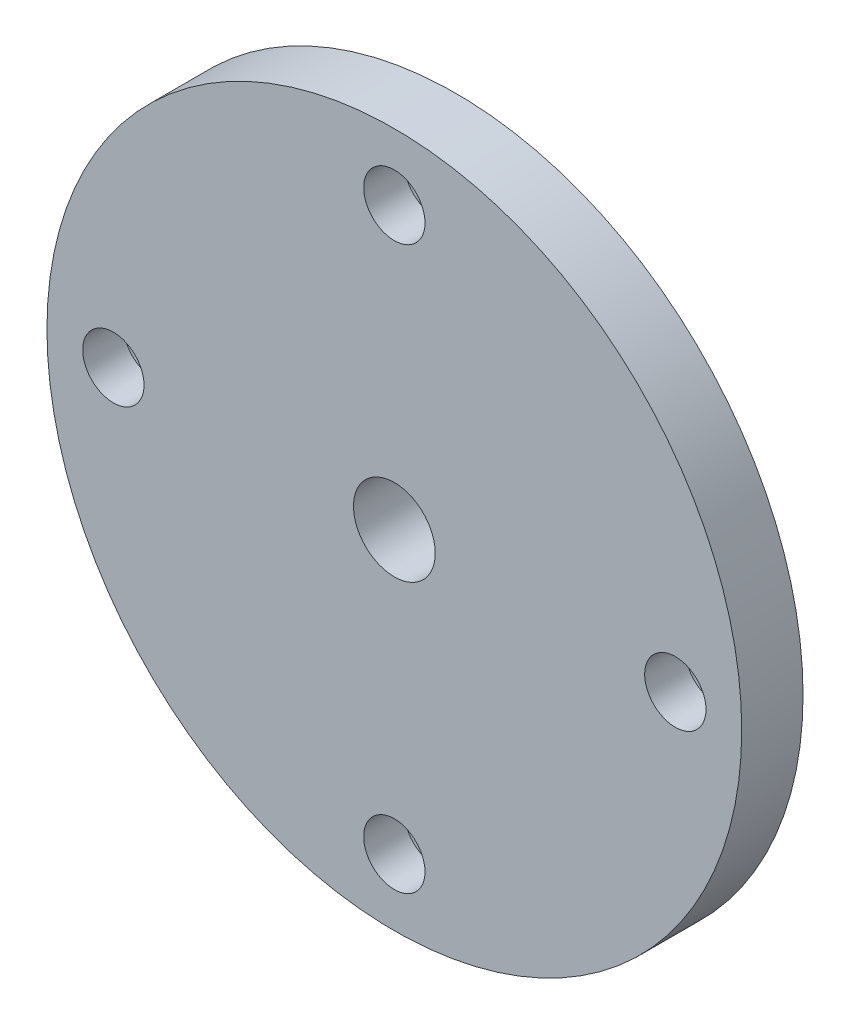
SolidWorks part; units mm, degrees
ref_plane "Front Plane" through (0, 0, 0) normal (0, 0, 1) x (1, 0, 0)
ref_plane "Top Plane" through (0, 0, 0) normal (0, 1, 0) x (1, 0, 0)
ref_plane "Right Plane" through (0, 0, 0) normal (1, 0, 0) x (0, 0, -1)
other "Configuration Table"
sketch "Sketch1" plane through (0, 0, 0) normal (0, 0, 1) x (1, 0, 0)
  circle A0 centre (0, 0) radius 34
  dimension "D1" = 68
extrude "Boss-Extrude1" add sketch "Sketch1" along normal blind 6
sketch "Sketch2" plane through (0, 0, 6) normal (0, 0, 1) x (1, 0, 0)
  circle A1 centre (0, 27.5) radius 3
  circle A3 centre (27.5, 0) radius 3
  circle A5 centre (0, -27.5) radius 3
  circle A7 centre (-27.5, 0) radius 3
  circle A9 centre (-19.4454, 19.4454) radius 3 [skipped]
  circle A10 centre (19.4454, 19.4454) radius 3 [skipped]
  circle A11 centre (19.4454, -19.4454) radius 3 [skipped]
  circle A12 centre (-19.4454, -19.4454) radius 3 [skipped]
  point P22 (0, 0)
  dimension "D1" = 27.5
  dimension "D2" = 6
  dimension "D3" = 8
extrude "Cut-Extrude1" cut sketch "Sketch2" against normal blind 4
sketch "Sketch3" plane through (0, 0, 6) normal (0, 0, 1) x (1, 0, 0)
  circle A0 centre (0, 0) radius 4
  dimension "D1" = 8
extrude "Cut-Extrude2" cut sketch "Sketch3" against normal through all
